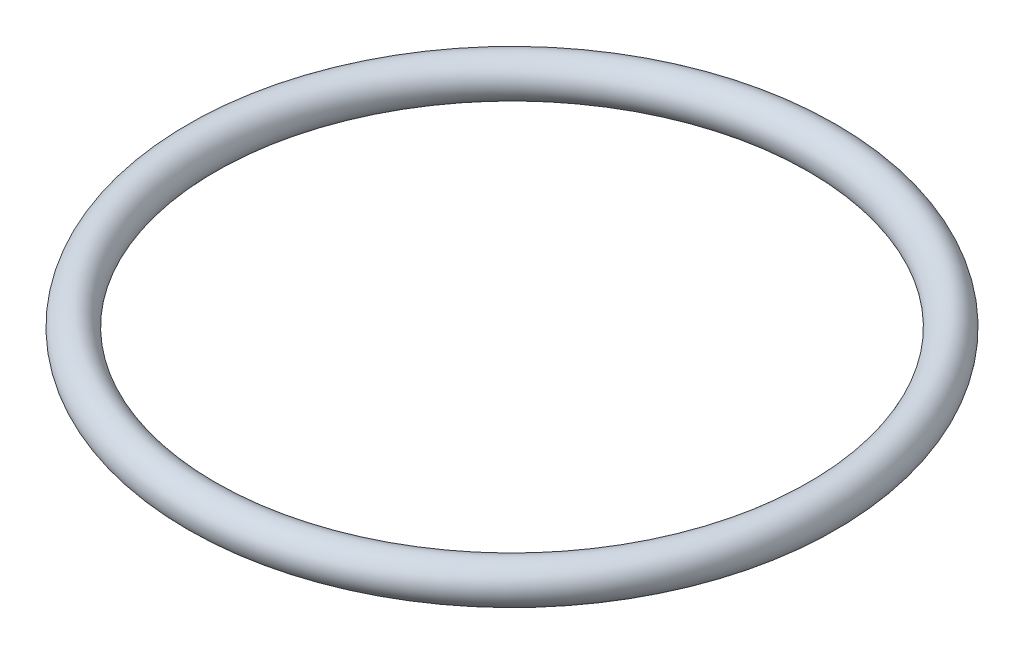
from build123d import *

# Parameters (mm, degrees)
SKETCH_1_R = 2.25


with BuildPart() as part:
    # 草图1 → 旋转1 (revolve)
    with BuildSketch(Plane.XY, mode=Mode.PRIVATE) as revolve_1_sk:
        with Locations((-36.125, 0)):
            Circle(SKETCH_1_R)
    revolve(revolve_1_sk.sketch.rotate(Axis((0, 0, 0), (0, 1, 0)), 270), axis=Axis((0, 0, 0), (0, 1, 0)))


solid = part.part
